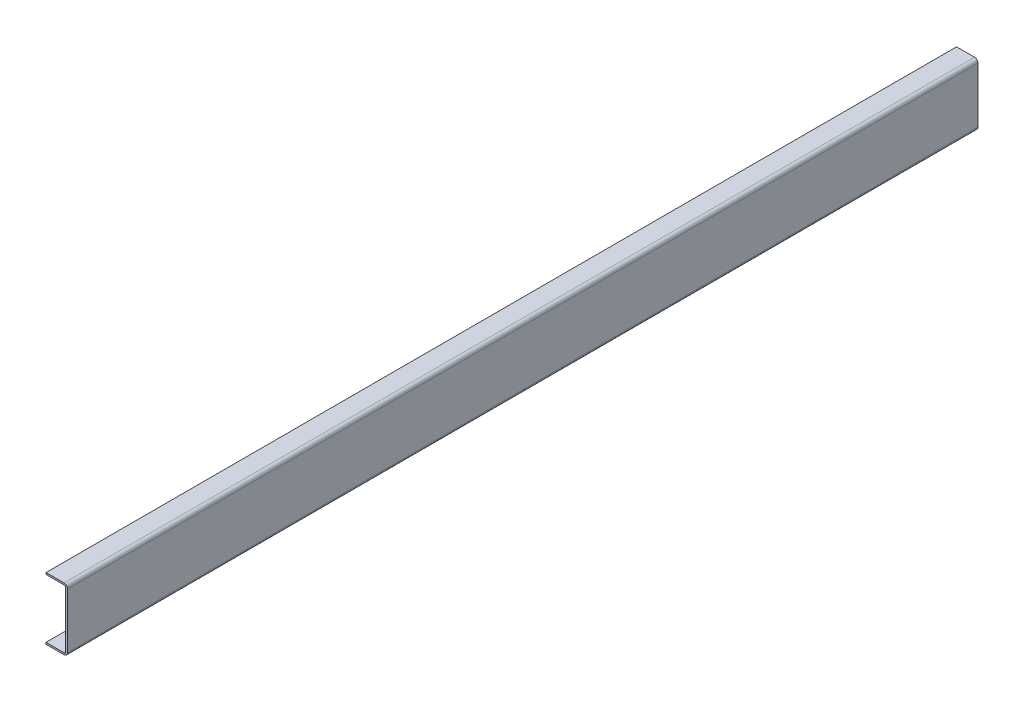
from build123d import *

# Parameters (mm, degrees)
BOSS_EXTRUDE1_DEPTH = 1062


with BuildPart() as part:
    # Sketch1 → Boss-Extrude1 (new, symmetric)
    with BuildSketch(Plane.XY):
        with BuildLine():
            Line((-50, -72.5), (-8, -72.5))
            ThreePointArc((-8, -72.5), (-2.343145751, -70.156854249), (0, -64.5))
            Line((0, -64.5), (0, 64.5))
            ThreePointArc((0, 64.5), (-2.343145751, 70.156854249), (-8, 72.5))
            Line((-8, 72.5), (-50, 72.5))
            Line((-50, 72.5), (-50, 68.5))
            Line((-50, 68.5), (-8, 68.5))
            ThreePointArc((-8, 68.5), (-5.171572875, 67.328427125), (-4, 64.5))
            Line((-4, 64.5), (-4, -64.5))
            ThreePointArc((-4, -64.5), (-5.171572875, -67.328427125), (-8, -68.5))
            Line((-8, -68.5), (-50, -68.5))
            Line((-50, -68.5), (-50, -72.5))
        make_face()
    extrude(amount=BOSS_EXTRUDE1_DEPTH, both=True)


solid = part.part
